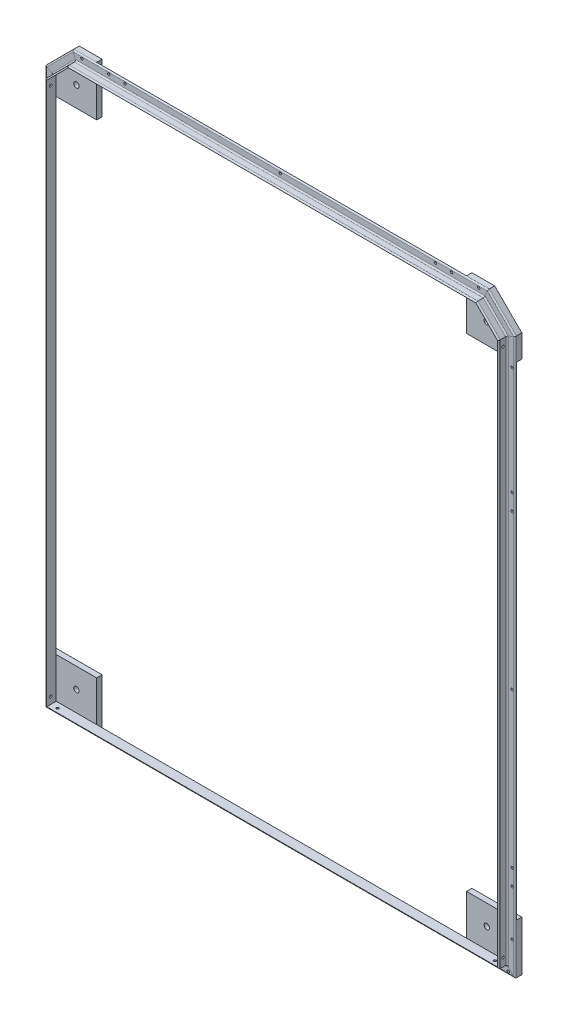
SolidWorks part; units mm, degrees
ref_plane "前视基准面" through (0, 0, 0) normal (0, 0, 1) x (1, 0, 0)
ref_plane "上视基准面" through (0, 0, 0) normal (0, 1, 0) x (1, 0, 0)
ref_plane "右视基准面" through (0, 0, 0) normal (1, 0, 0) x (0, 0, -1)
sketch "草图1" plane through (0, 0, 0) normal (0, 0, 1) x (1, 0, 0)
  line L0 (0, 2010) -> (80, 2090)
  line L1 (0, 0) -> (1670, 0)
  line L2 (0, 0) -> (0, 2010)
  line L3 (80, 2090) -> (1590, 2090)
  line L4 (1670, 0) -> (1670, 2010)
  line L5 (1590, 2090) -> (1670, 2010)
  point P1 (1670, 2090)
  point P2 (0, 2090)
  dimension "D1" = 1670
  dimension "D2" = 2090
other "结构构件1"
ref_plane "基准面1" through (0, 0, 0) normal (0, 1, 0) x (-1, 0, 0)
sketch "Sketch1" plane through (0, 0, 0) normal (0, 1, 0) x (-1, 0, 0)
  line L0 (0, 0) -> (0, 35)
  line L1 (0, 17.5) -> (5, 17.5) construction
  line L2 (5, 30) -> (5, 10)
  line L3 (10, 5) -> (30, 5)
  line L4 (17.5, 5) -> (17.5, 0) construction
  line L5 (35, 0) -> (0, 0)
  arc A0 (35, 0) -> (30, 5) centre (30, 0) ccw
  arc A1 (0, 35) -> (5, 30) centre (0, 30) cw
  arc A2 (10, 5) -> (5, 10) centre (10, 10) cw
  point P10 (17.5, 0)
  point P14 (0, 17.5)
  point P15 (5, 17.5)
  point P16 (17.5, 5)
  point P17 (5, 35)
  point P18 (35, 5)
  point P21 (0, 0)
  dimension "D2" = 5
  dimension "D3" = 35
  dimension "Radius_1" = 5
  dimension "D1" = 5
sketch "草图3" plane through (0, 0, 0) normal (0, 0, -1) x (-1, 0, 0)
  line L0 (-1604.4975, 2125) -> (-1705, 2024.4975)
  line L1 (-1705, 2024.4975) -> (-1705, 1940)
  line L2 (-1705, -35) -> (-1705, 2024.4975) construction
  line L3 (-1705, 1940) -> (-1520, 1940)
  line L4 (-1520, 1940) -> (-1520, 2125)
  line L5 (-1604.4975, 2125) -> (-65.5025, 2125) construction
  line L6 (-80, 2090) -> (-1590, 2090) construction
  line L7 (-1520, 2125) -> (-1604.4975, 2125)
  line L8 (-1590, 2090) -> (-80, 2090) construction
  line L10 (-1670, 0) -> (-1670, 2010) construction
  line L11 (-835, 2090) -> (-835, -202.4878) construction
  line L12 (0, 0) -> (-1670, 0) construction
  line L13 (-1705, -35) -> (-1520, -35)
  line L14 (-1705, -35) -> (-1705, 150)
  line L15 (-1705, 150) -> (-1520, 150)
  line L16 (-1520, -35) -> (-1520, 150)
  line L17 (-150, -35) -> (-150, 150)
  line L18 (35, 150) -> (-150, 150)
  line L19 (35, -35) -> (35, 150)
  line L20 (35, -35) -> (-150, -35)
  line L21 (-150, 2125) -> (-65.5025, 2125)
  line L22 (-150, 1940) -> (-150, 2125)
  line L23 (35, 1940) -> (-150, 1940)
  line L24 (35, 2024.4975) -> (35, 1940)
  line L25 (-65.5025, 2125) -> (35, 2024.4975)
  circle A0 centre (-1595, 2015) radius 10
  circle A1 centre (-1595, 75) radius 10
  circle A2 centre (-75, 75) radius 10
  circle A3 centre (-75, 2015) radius 10
  dimension "D3" = 20
  dimension "D4" = 75
  dimension "D5" = 75
  dimension "D8" = 20
  dimension "D9" = 75
  dimension "D10" = 75
  dimension "D1" = 150
  dimension "D2" = 150
  dimension "D6" = 150
  dimension "D7" = 150
extrude "凸台-拉伸1" add sketch "草图3" along normal blind 20 separate body
sketch "草图4" plane through (0, 0, 0) normal (0, 1, 0) x (1, 0, 0)
  line L0 (835, 0) -> (835, -419.2176) construction
  line L1 (1604.4975, 0) -> (65.5025, 0) construction
  line L2 (65.5025, 0) -> (150, 0) construction
  circle A0 centre (25, -20) radius 4.5
  circle A1 centre (1645, -20) radius 4.5
  dimension "D1" = 9
  dimension "D2" = 20
  dimension "D3" = 810
extrude "切除-拉伸1" cut sketch "草图4" against normal blind 10
sketch "草图5" plane through (0, 0, 0) normal (1, 0, 0) x (0, 0, -1)
  line L0 (-35, 1005) -> (207.0048, 1005) construction
  line L1 (-35, 2010) -> (-35, 0) construction
  line L2 (0, 2010) -> (0, 0) construction
  circle A0 centre (-20, 25) radius 4.5
  circle A1 centre (-20, 1985) radius 4.5
  dimension "D1" = 9
  dimension "D2" = 20
  dimension "D3" = 980
extrude "切除-拉伸2" cut sketch "草图5" against normal blind 328 and the other way blind 2262
sketch "草图6" plane through (0, 0, 5) normal (0, 0, 1) x (1, 0, 0)
  line L50 (1590, 2090) -> (80, 2090) construction
  line L51 (0, 2010) -> (0, 0) construction
  line L52 (835, 2114) -> (835, -388.9414) construction
  line L56 (-24, -24) -> (1694, -24)
  line L57 (1694, -24) -> (1694, 2019.9411)
  line L58 (1694, 2019.9411) -> (1599.9411, 2114)
  line L59 (-24, 2019.9411) -> (-24, -24)
  line L60 (70.0589, 2114) -> (-24, 2019.9411)
  line L61 (1599.9411, 2114) -> (70.0589, 2114)
  line L62 (-24, -24) -> (1694, -24) construction
  line L63 (1694, -24) -> (1694, 2019.9411) construction
  line L64 (1694, 2019.9411) -> (1599.9411, 2114) construction
  line L65 (-24, 2019.9411) -> (-24, -24) construction
  line L66 (70.0589, 2114) -> (-24, 2019.9411) construction
  line L67 (1599.9411, 2114) -> (70.0589, 2114) construction
  circle A0 centre (100, 2114) radius 4.5
  circle A1 centre (200, 2114) radius 4.5
  circle A2 centre (-24, 1920) radius 4.5
  circle A3 centre (-24, 1790) radius 4.5
  circle A4 centre (1470, 2114) radius 4.5
  circle A5 centre (1570, 2114) radius 4.5
  circle A6 centre (1694, 1920) radius 4.5
  circle A7 centre (1694, 1519) radius 4.5
  circle A8 centre (260, 2114) radius 4.5
  circle A9 centre (835, 2114) radius 4.5
  circle A10 centre (1410, 2114) radius 4.5
  dimension "D2" = 9
  dimension "D3" = 9
  dimension "D4" = 9
  dimension "D5" = 9
  dimension "D8" = 100
  dimension "D9" = 200
  dimension "D10" = 9
  dimension "D11" = 571
  dimension "D12" = 9
  dimension "D13" = 9
  dimension "D14" = 260
  dimension "D6" = 170
  dimension "D7" = 300
  dimension "D1" = 24
extrude "切除-拉伸3" cut sketch "草图6" against normal blind 236
sketch "草图7" plane through (0, 0, 5) normal (0, 0, 1) x (1, 0, 0)
  line L0 (-24, 392.516) -> (-24, -118.4613) construction
  line L1 (-79.6135, -24) -> (377.1095, -24) construction
  line L2 (-35, 2024.4975) -> (-35, -35) construction
  line L3 (150, -35) -> (-35, -35) construction
  line L4 (0, 0) -> (1670, 0) construction
  line L5 (0, 2010) -> (0, 0) construction
  circle A0 centre (-24, 73) radius 4.5
  circle A1 centre (-24, 273) radius 4.5
  circle A2 centre (80, -24) radius 4.5
  point P6 (57.5, -35)
  dimension "D4" = 273
  dimension "D5" = 80
  dimension "D6" = 9
  dimension "D7" = 9
  dimension "D8" = 9
  dimension "D1" = 11
  dimension "D2" = 11
  dimension "D3" = 73
extrude "切除-拉伸4" cut sketch "草图7" against normal blind 228
sketch "草图8" plane through (0, 0, 5) normal (0, 0, 1) x (1, 0, 0)
  line L0 (1694, 1823.5276) -> (1694, -91.3206) construction
  line L1 (1705, -35) -> (1705, 2024.4975) construction
  line L2 (0, 0) -> (1670, 0) construction
  circle A0 centre (1694, 255) radius 4.5
  circle A1 centre (1694, 85) radius 4.5
  circle A2 centre (1694, 315) radius 4.5
  circle A3 centre (1694, 887) radius 4.5
  circle A4 centre (1694, 1459) radius 4.5
  dimension "D2" = 9
  dimension "D3" = 9
  dimension "D4" = 255
  dimension "D5" = 85
  dimension "D6" = 9
  dimension "D7" = 9
  dimension "D8" = 9
  dimension "D9" = 1144
  dimension "D10" = 315
  dimension "D1" = 11
  dimension "D11" = 887
extrude "切除-拉伸5" cut sketch "草图8" against normal blind 99
sketch "草图9" plane through (0, 0, 5) normal (0, 0, 1) x (1, 0, 0)
  line L1 (1670, 0) -> (1670, 2010) construction
  line L2 (0, -24) -> (1670, -24)
  line L3 (0, -24) -> (1799.5581, -24) construction
  circle A0 centre (1680, -24) radius 4.5
  circle A1 centre (140, -24) radius 4.5
  circle A2 centre (910, -24) radius 4.5
  dimension "D3" = 9
  dimension "D4" = 9
  dimension "D5" = 9
  dimension "D6" = 1540
  dimension "D7" = 770
  dimension "D2" = 10
  dimension "D1" = 24
extrude "切除-拉伸6" cut sketch "草图9" against normal blind 78
